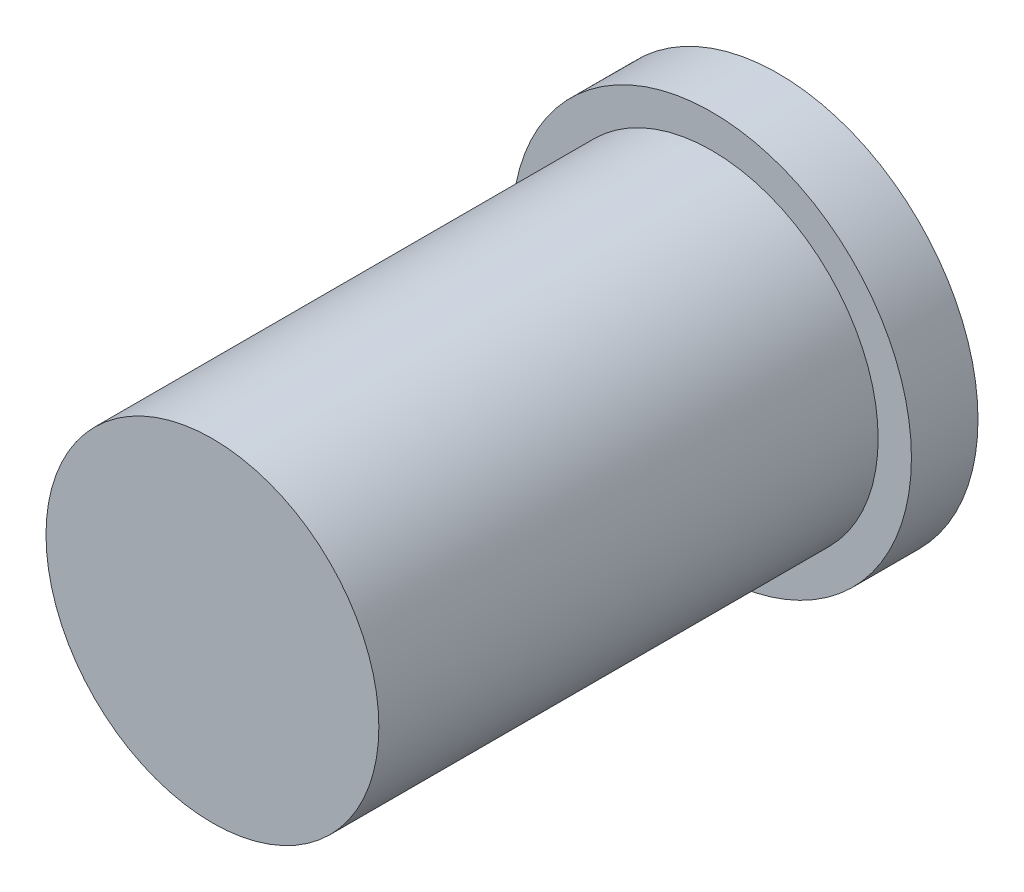
SolidWorks part; units mm, degrees
ref_plane "Front Plane" through (0, 0, 0) normal (0, 0, 1) x (1, 0, 0)
ref_plane "Top Plane" through (0, 0, 0) normal (0, 1, 0) x (1, 0, 0)
ref_plane "Right Plane" through (0, 0, 0) normal (1, 0, 0) x (0, 0, -1)
other "Configuration Table"
sketch "Sketch1" plane through (0, 0, 0) normal (0, 0, 1) x (1, 0, 0)
  circle A0 centre (0, 0) radius 6
  dimension "D1" = 12
extrude "Boss-Extrude1" add sketch "Sketch1" along normal blind 2
sketch "Sketch2" plane through (0, 0, 2) normal (0, 0, 1) x (1, 0, 0)
  circle A0 centre (0, 0) radius 5
  dimension "D1" = 10
extrude "Boss-Extrude2" add sketch "Sketch2" along normal blind 15
